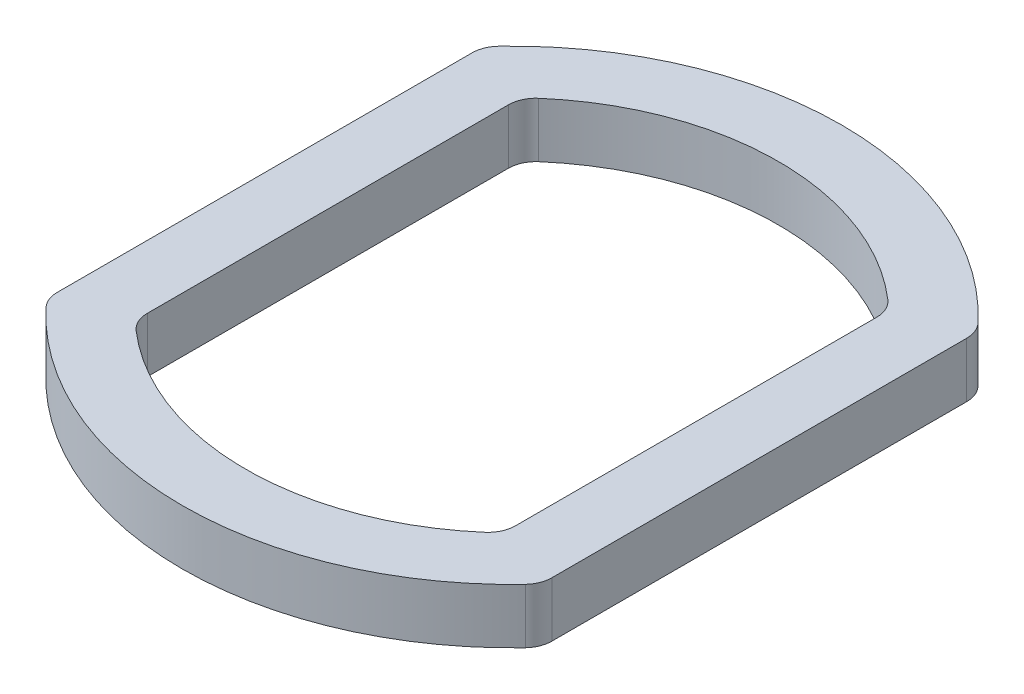
from build123d import *

# Parameters (mm, degrees)
EXTRUDE_1_DEPTH = 20
FILLET_1_R      = 10


with BuildPart() as part:
    # 草图1 → 凸台-拉伸1 (new body)
    with BuildSketch(Plane(origin=(0, 0, 0), x_dir=(1, 0, 0), z_dir=(0, 1, 0))):
        with BuildLine():
            Line((90, -75.498344353), (90, 75.498344353))
            ThreePointArc((90, 75.498344353), (89.293203773, 79.191089082), (87.272727273, 82.361830203))
            ThreePointArc((87.272727273, 82.361830203), (0, 120), (-87.272727273, 82.361830203))
            ThreePointArc((-87.272727273, 82.361830203), (-89.293203773, 79.191089082), (-90, 75.498344353))
            Line((-90, 75.498344353), (-90, -75.498344353))
            ThreePointArc((-90, -75.498344353), (-89.293203773, -79.191089082), (-87.272727273, -82.361830203))
            ThreePointArc((-87.272727273, -82.361830203), (0, -120), (87.272727273, -82.361830203))
            ThreePointArc((87.272727273, -82.361830203), (89.293203773, -79.191089082), (90, -75.498344353))
        make_face()
        with BuildLine():
            Line((67, -70.142711667), (67, 70.142711667))
            ThreePointArc((67, 70.142711667), (0, 97), (-67, 70.142711667))
            Line((-67, 70.142711667), (-67, -70.142711667))
            ThreePointArc((-67, -70.142711667), (0, -97), (67, -70.142711667))
        make_face(mode=Mode.SUBTRACT)
    extrude(amount=EXTRUDE_1_DEPTH)

    # 圆角1
    fillet_1_edges = [part.edges().sort_by_distance(p)[0] for p in [
        (-67, 10, 70.142711667),
        (67, 10, 70.142711667),
        (67, 10, -70.142711667),
        (-67, 10, -70.142711667),
    ]]
    fillet(fillet_1_edges, radius=FILLET_1_R)


solid = part.part
